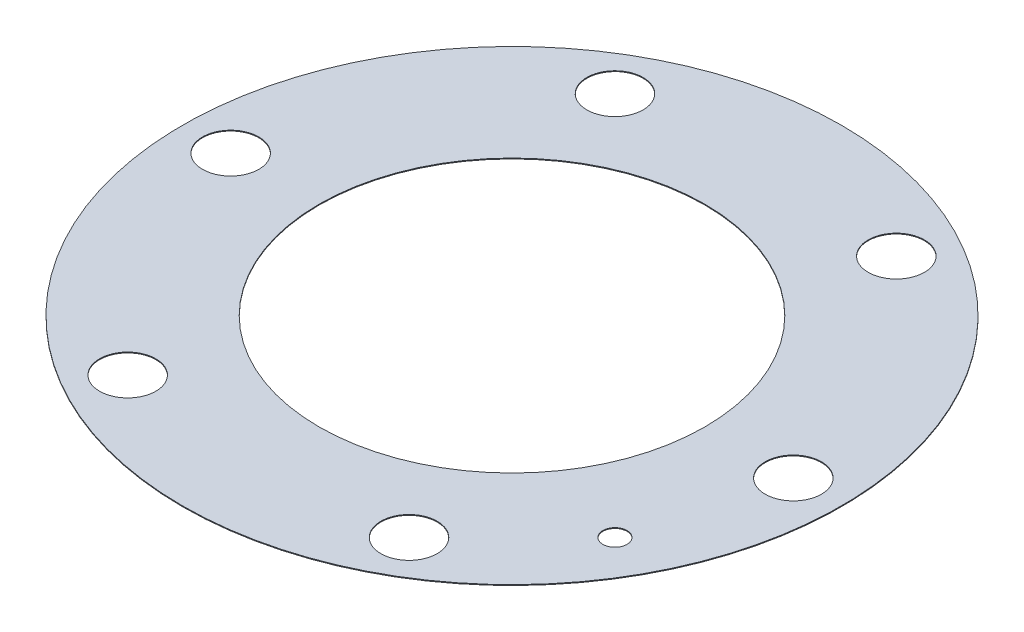
SolidWorks part; units mm, degrees
ref_plane "Front Plane" through (0, 0, 0) normal (0, 0, 1) x (1, 0, 0)
ref_plane "Top Plane" through (0, 0, 0) normal (0, 1, 0) x (1, 0, 0)
ref_plane "Right Plane" through (0, 0, 0) normal (1, 0, 0) x (0, 0, -1)
other "Configuration Table"
sketch "Sketch1" plane through (0, 0, 0) normal (0, 1, 0) x (1, 0, 0)
  line L0 (-64.2909, 0) -> (76.9146, 0) construction
  line L1 (0, 49.999) -> (0, -46.3399) construction
  line L2 (0, 0) -> (47.3315, -27.3268) construction
  circle A0 centre (0, 0) radius 24
  circle A1 centre (0, 0) radius 35 construction
  circle A2 centre (0, 0) radius 41
  circle A3 centre (35, 0) radius 3.5
  circle A4 centre (17.5, -30.3109) radius 3.5
  circle A5 centre (-17.5, -30.3109) radius 3.5
  circle A6 centre (-35, 0) radius 3.5
  circle A7 centre (-17.5, 30.3109) radius 3.5
  circle A8 centre (17.5, 30.3109) radius 3.5
  circle A9 centre (30.3109, -17.5) radius 1.5
  point P23 (0, 0)
  dimension "D1" = 82
  dimension "D2" = 70
  dimension "D3" = 48
  dimension "D4" = 7
  dimension "D6" = 3
  dimension "D5" = 30
extrude "Boss-Extrude1" add sketch "Sketch1" along normal blind 0.1
